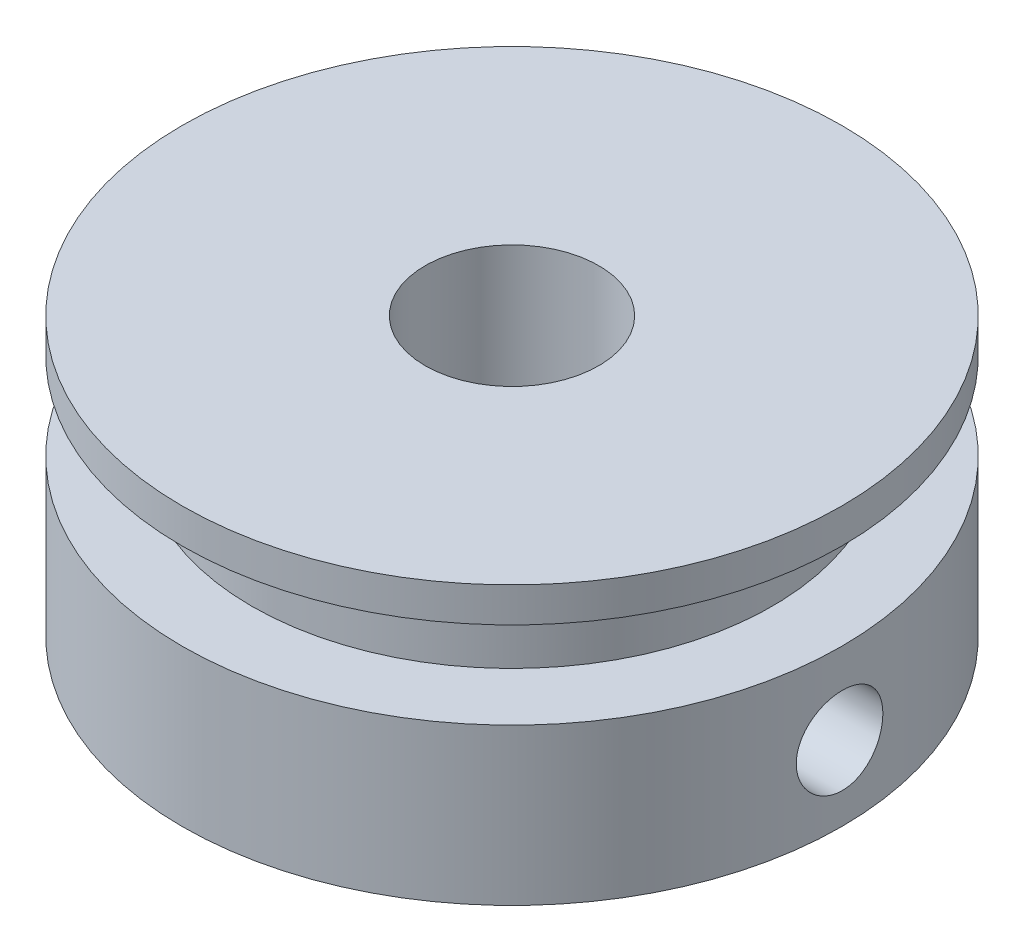
from build123d import *

# Parameters (mm, degrees)
HOLE_WIZARD_M3_1_REACH  = 24.044
HOLE_WIZARD_M3_1_BORE_R = 1.25


with BuildPart() as part:
    # 草图1 → 旋转1 (revolve)
    with BuildSketch(Plane.XY, mode=Mode.PRIVATE) as revolve_1_sk:
        Polygon((2.5, 4), (2.5, -4), (9.5, -4), (9.5, 0.5), (7.5, 0.5), (7.5, 3), (9.5, 3), (9.5, 4), align=None)
    revolve(revolve_1_sk.sketch.rotate(Axis((0, 34.071946617, 0), (0, -1, 0)), 90), axis=Axis((0, 34.071946617, 0), (0, -1, 0)))

    # M3 螺纹孔1 bore (on position points) → M3 螺纹孔1 (cut, up to next)
    with BuildSketch(Plane(origin=(9.499977586, -1.857282502, -0.020636472), x_dir=(0.002172260237, 0, 0.99999764064), z_dir=(0.99999764064, 0, -0.002172260237)), mode=Mode.PRIVATE) as hole_wizard_m3_1_sk1:
        Circle(HOLE_WIZARD_M3_1_BORE_R)
    hole_wizard_m3_1_tool1 = extrude(hole_wizard_m3_1_sk1.sketch, amount=-HOLE_WIZARD_M3_1_REACH, mode=Mode.PRIVATE) & part.part
    add(hole_wizard_m3_1_tool1.solids().sort_by_distance((9.499978, -1.857283, -0.020636))[0], mode=Mode.SUBTRACT)


solid = part.part
